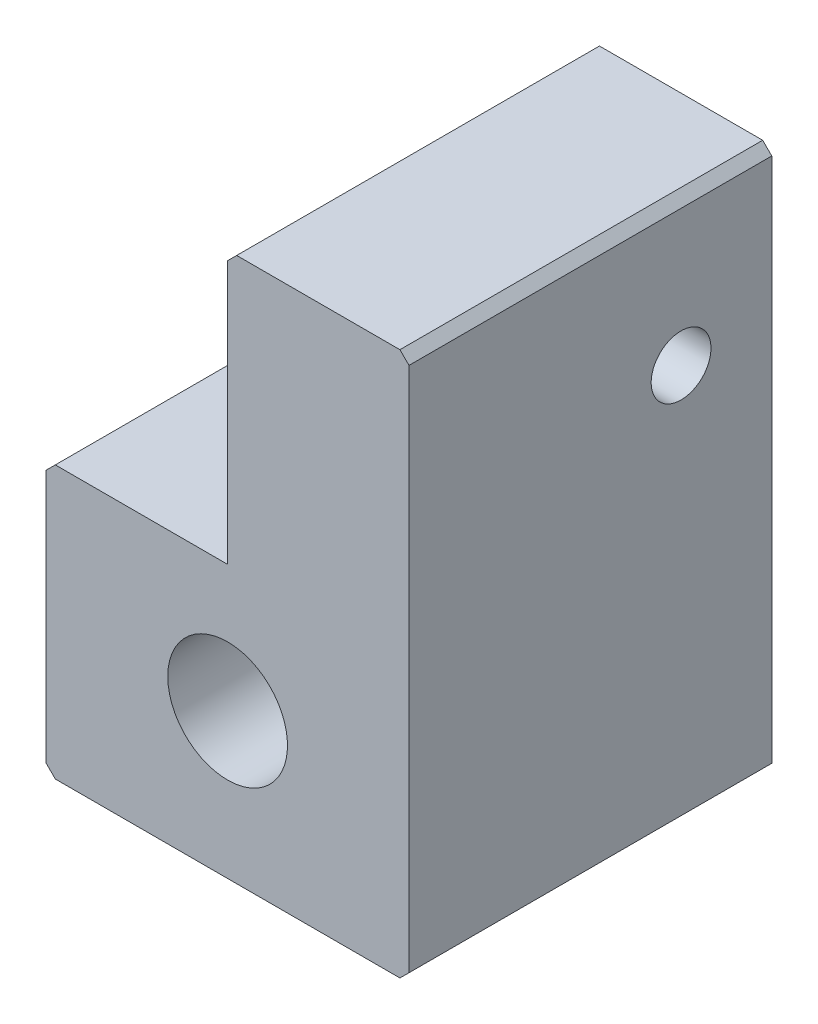
from build123d import *

# Parameters (mm, degrees)
SKETCH_1_W                = 20
SKETCH_1_H                = 30
EXTRUDE_1_DEPTH           = 20
HOLE_WIZARD_1_D           = 6.6
HOLE_WIZARD_1_CBORE_D     = 11
HOLE_WIZARD_1_CBORE_DEPTH = 6.8
SKETCH_4_W                = 10
SKETCH_4_H                = 15
CUT_EXTRUDE_1_DEPTH       = 27.925824036
HOLE_WIZARD_M4_1_D        = 3.3
CHAMFER_1_SIZE            = 0.5


with BuildPart() as part:
    # 草图1 → 凸台-拉伸1 (new body)
    with BuildSketch(Plane.XY):
        Rectangle(SKETCH_1_W, SKETCH_1_H)
    extrude(amount=EXTRUDE_1_DEPTH)

    # 打孔尺寸根据内六角圆柱头螺钉的类型1 (through all)
    with Locations(Plane(origin=(3.133596483, 10.907898158, 0), x_dir=(1, 0, 0), z_dir=(0, 0, -1))):
        with Locations((-3.133596483, 17.907898158)):
            CounterBoreHole(HOLE_WIZARD_1_D / 2, HOLE_WIZARD_1_CBORE_D / 2, HOLE_WIZARD_1_CBORE_DEPTH)

    # 草图4 → 切除-拉伸1 (cut, through all)
    with BuildSketch(Plane.XY.offset(20)):
        with Locations((-5, 7.5)):
            Rectangle(SKETCH_4_W, SKETCH_4_H)
    extrude(amount=-CUT_EXTRUDE_1_DEPTH, mode=Mode.SUBTRACT)

    # M4 螺纹孔1 (through all)
    with Locations(Plane.ZY):
        with Locations((5, 7)):
            Hole(HOLE_WIZARD_M4_1_D / 2)

    # 倒角1
    chamfer_1_edges = [part.edges().sort_by_distance(p)[0] for p in [
        (-10, 0, 10),
        (0, 15, 10),
        (10, -15, 10),
        (-10, -15, 10),
        (10, 15, 10),
    ]]
    chamfer(chamfer_1_edges, length=CHAMFER_1_SIZE)


solid = part.part
